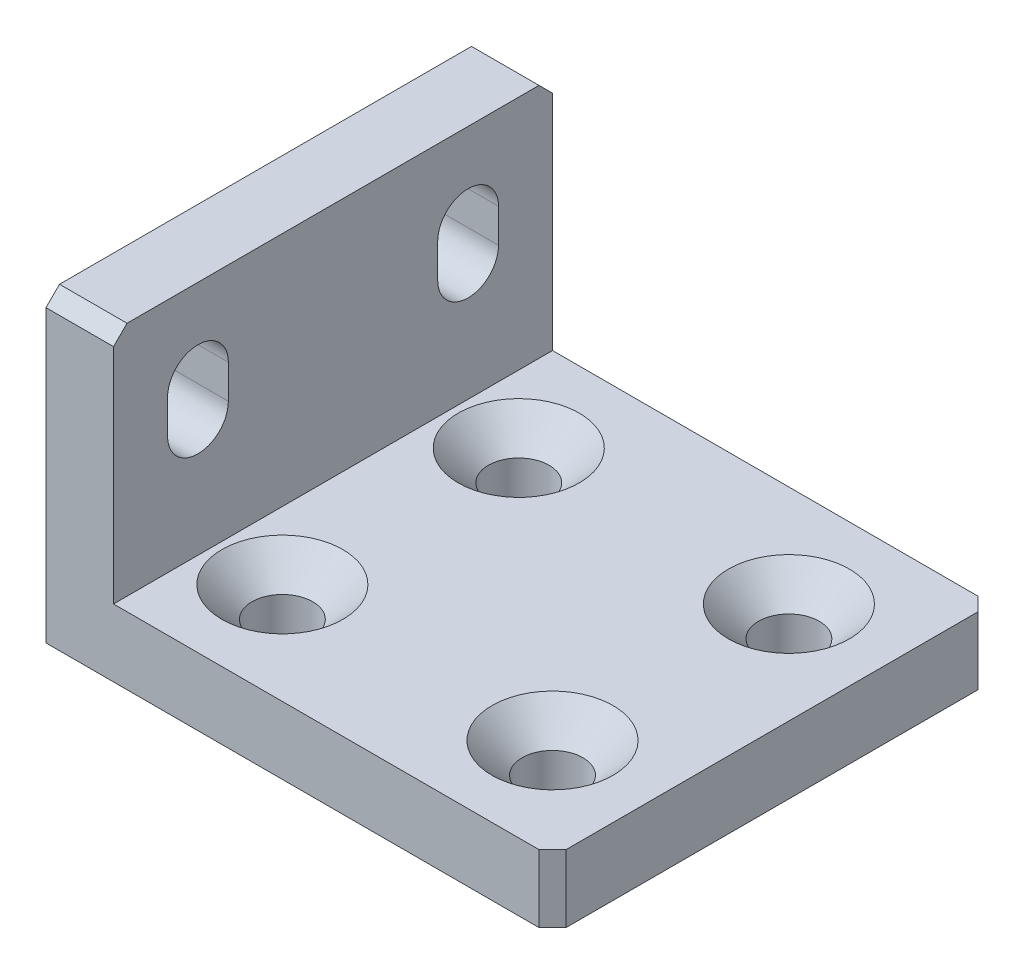
SolidWorks part; units mm, degrees
ref_plane "前视基准面" through (0, 0, 0) normal (0, 0, 1) x (1, 0, 0)
ref_plane "上视基准面" through (0, 0, 0) normal (0, 1, 0) x (1, 0, 0)
ref_plane "右视基准面" through (0, 0, 0) normal (1, 0, 0) x (0, 0, -1)
sketch "草图2" plane through (0, 0, 0) normal (0, 1, 0) x (1, 0, 0)
  line L1 (-37.5, 32.5) -> (37.5, 32.5)
  line L2 (-37.5, 32.5) -> (-37.5, -32.5)
  line L3 (-37.5, -32.5) -> (37.5, -32.5)
  line L4 (37.5, 32.5) -> (37.5, -32.5)
  line L5 (-37.5, 32.5) -> (37.5, -32.5) construction
  line L6 (-37.5, -32.5) -> (37.5, 32.5) construction
  point P0 (0, 0)
  dimension "D1" = 75
  dimension "D2" = 65
extrude "凸台-拉伸1" add sketch "草图2" along normal mid plane 10
sketch "草图3" plane through (0, -5, 0) normal (0, -1, 0) x (1, 0, 0)
  line L0 (-37.5, 32.5) -> (37.5, 32.5) construction
  line L1 (-37.5, -32.5) -> (-27.5, -32.5)
  line L2 (-37.5, -32.5) -> (-37.5, 32.5)
  line L3 (-37.5, 32.5) -> (-27.5, 32.5)
  line L4 (-27.5, -32.5) -> (-27.5, 32.5)
  dimension "D1" = 10
extrude "凸台-拉伸2" add sketch "草图3" against normal blind 45 contours L4 L3 L2 L1
hole_wizard "M8 六角凹锥坑螺钉的锥形沉头孔1" positions "草图5" profile "草图4" countersink size "M8" standard "ISO" end condition through all
sketch "草图5" plane through (0, 5, 0) normal (0, 1, 0) x (1, 0, 0)
  line L0 (37.5, -32.5) -> (37.5, 32.5) construction
  line L1 (-8.6595, 0) -> (13.4751, 0) construction
  point P0 (22.5, 17.5)
  point P2 (-17.5, 17.5)
  point P12 (-17.5, -17.5)
  point P13 (22.5, -17.5)
  dimension "D1" = 15
  dimension "D2" = 40
  dimension "D3" = 35
sketch "草图4" plane through (22.5, 5, -17.5) normal (1, 0, 0) x (0, 0, 1)
  line L0 (0, 0) -> (0, 10)
  line L1 (0, 10) -> (4.5, 10)
  line L2 (4.5, 10) -> (4.5, 4.46)
  line L3 (4.5, 4.46) -> (8.96, 0)
  line L5 (8.96, 0) -> (0, 0)
  line L6 (-4.5, 4.46) -> (-8.96, 0) construction
  line L11 (0, -6.35) -> (0, 107.95) construction
  dimension "通孔孔直径" = 9
  dimension "通孔孔深度" = 10
  dimension "近端锥形沉头孔直径" = 17.92
  dimension "近端锥形沉头孔角度" = 90
sketch "草图6" plane through (-27.5, 0, 0) normal (1, 0, 0) x (0, 0, -1)
  line L0 (20, 27.5) -> (20, 22.5) construction
  line L1 (24.5, 27.5) -> (24.5, 22.5)
  line L2 (15.5, 27.5) -> (15.5, 22.5)
  line L4 (0, 0) -> (0, 36.2035) construction
  line L5 (-20, 27.5) -> (-20, 22.5) construction
  line L6 (-24.5, 27.5) -> (-24.5, 22.5)
  line L7 (-15.5, 27.5) -> (-15.5, 22.5)
  line L8 (32.5, 40) -> (-32.5, 40) construction
  arc A0 (24.5, 27.5) -> (15.5, 27.5) centre (20, 27.5) ccw
  arc A1 (15.5, 22.5) -> (24.5, 22.5) centre (20, 22.5) ccw
  arc A2 (-24.5, 27.5) -> (-15.5, 27.5) centre (-20, 27.5) cw
  arc A3 (-15.5, 22.5) -> (-24.5, 22.5) centre (-20, 22.5) cw
  point P2 (20, 25)
  point P14 (-20, 25)
  dimension "D1" = 9
  dimension "D2" = 5
  dimension "D3" = 15
  dimension "D4" = 20
extrude "切除-拉伸1" cut sketch "草图6" against normal blind 45
chamfer "倒角1" distance 2 angle 45 4 edges at (37.5, 0, 32.5) (37.5, 0, -32.5) (-32.5, 40, -32.5) (-32.5, 40, 32.5)
